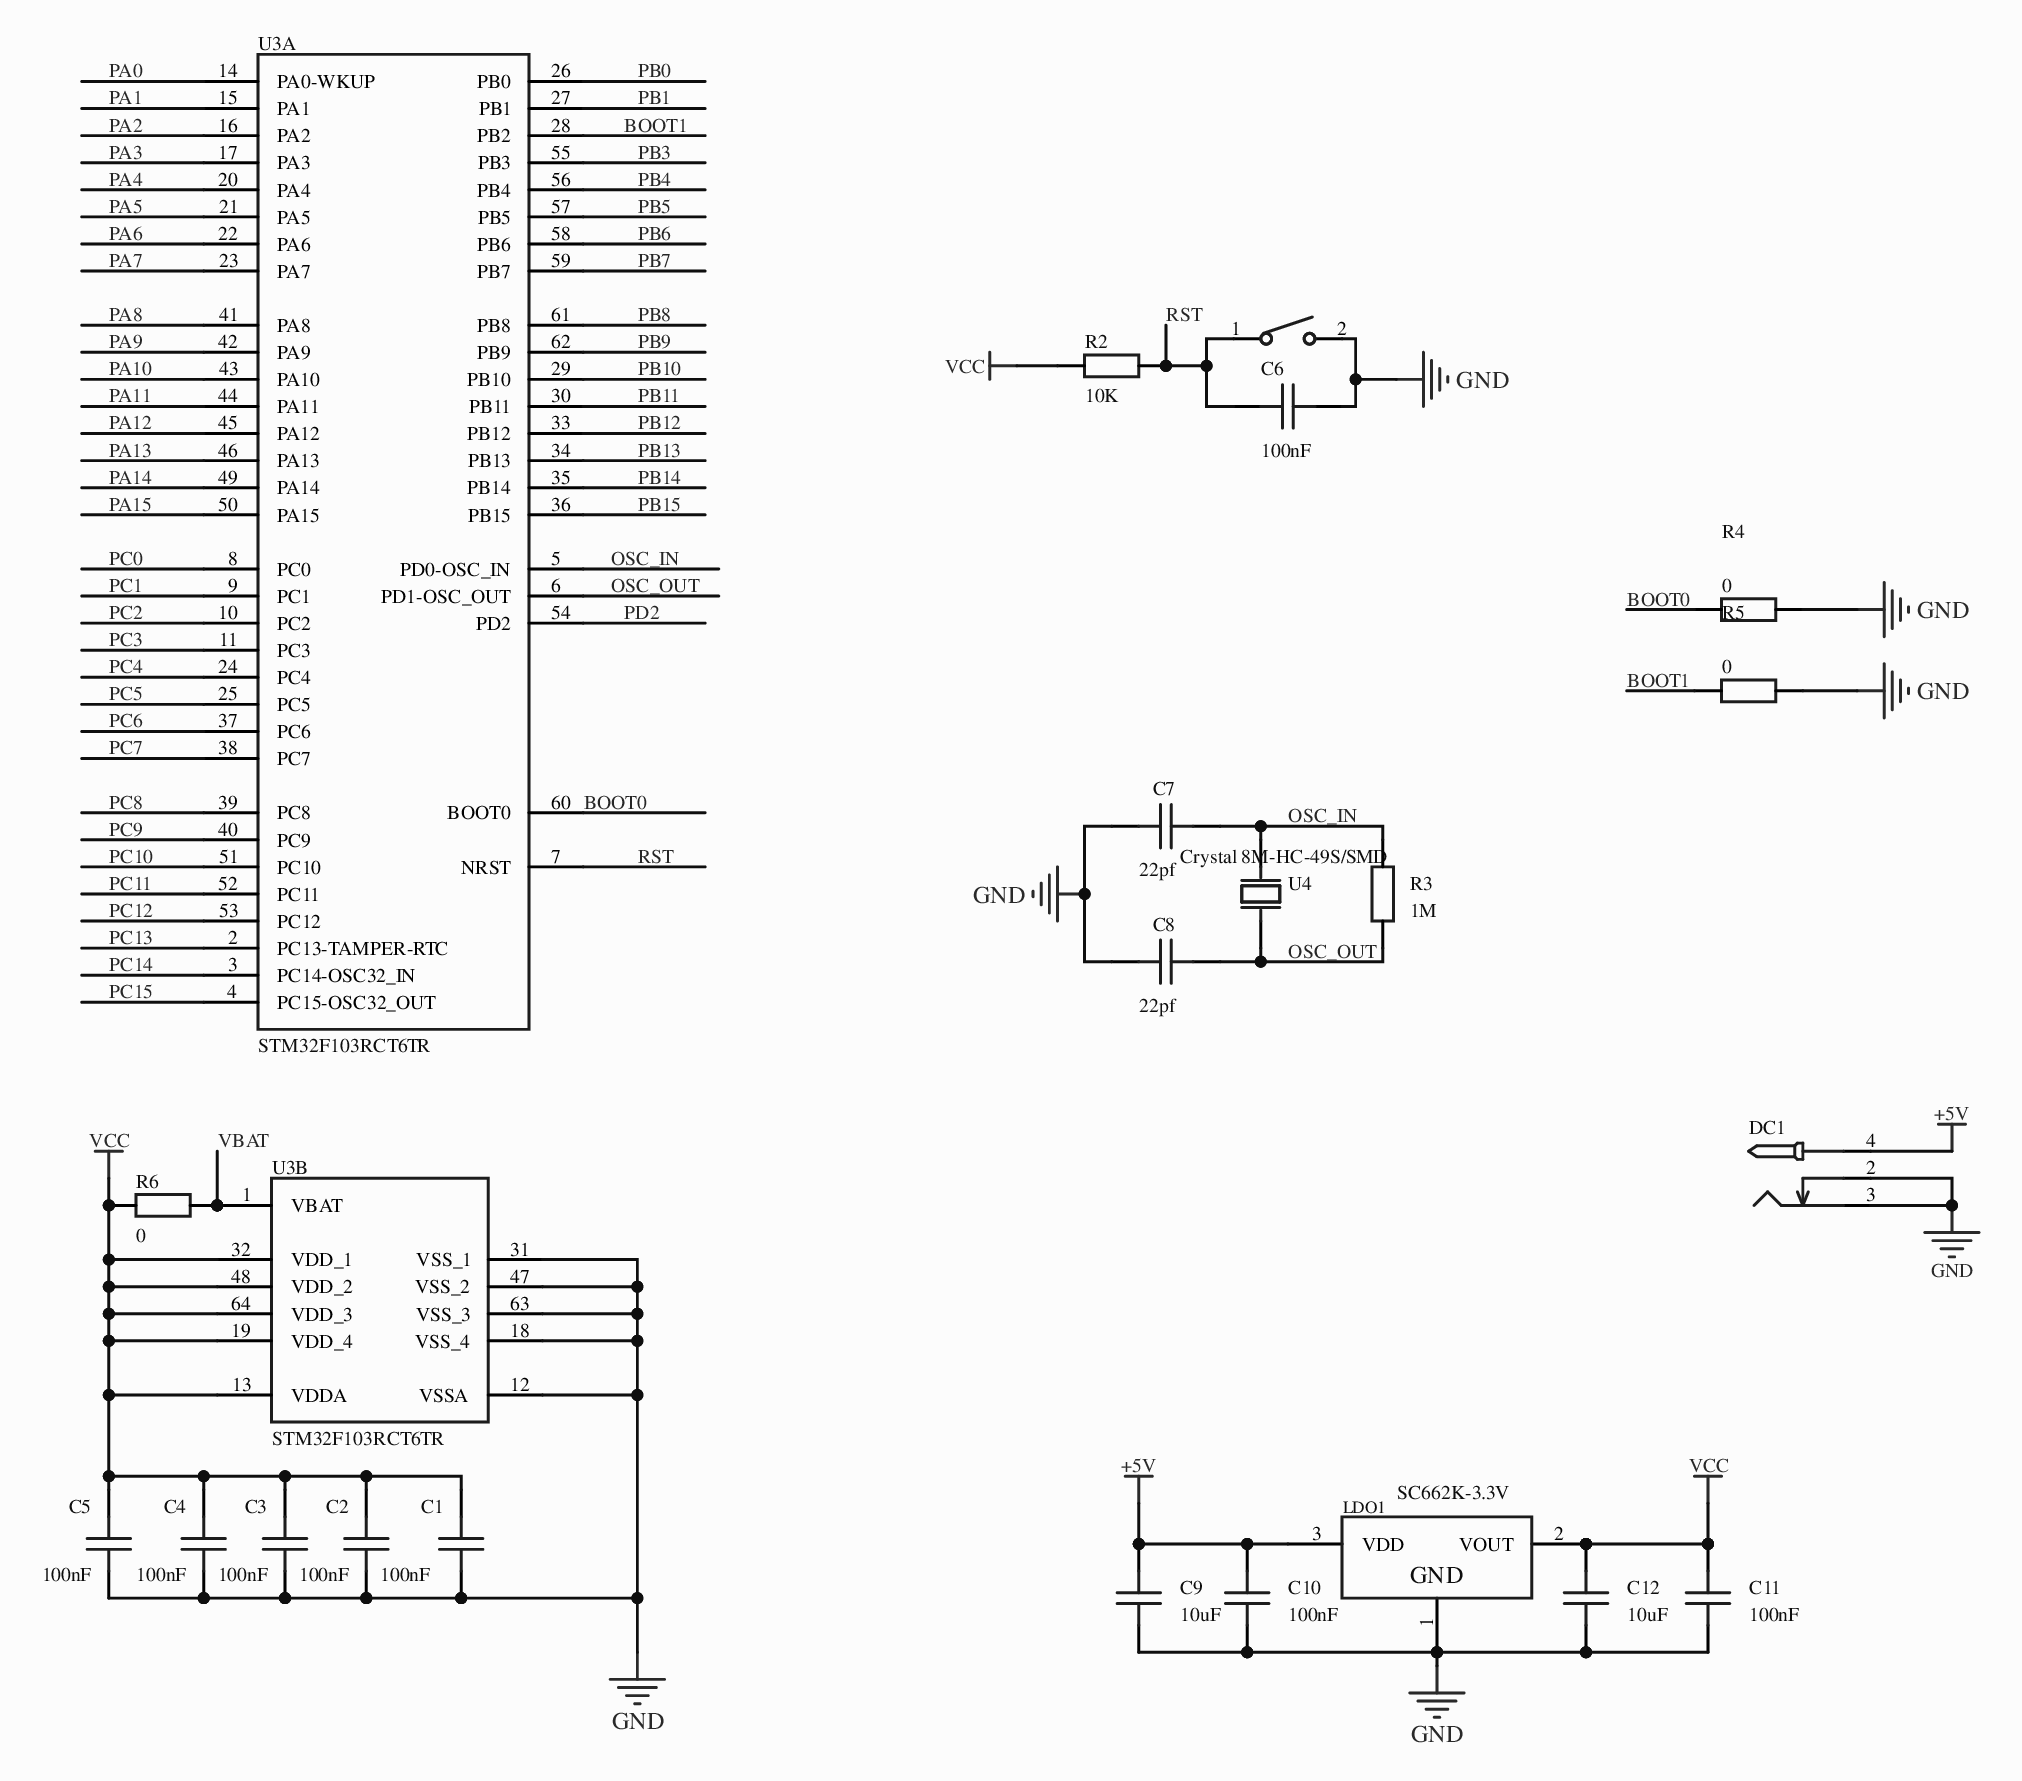
[diagram p0: MISC52126-3.schdoc]
# Altium project MISC52126-2.PrjPcb
1 sheet, 22 parts. Net scope: global (net labels, ports and power ports of the same name join across sheets).
Board file: MISC52126.pcbdoc

## Sheet MISC52126-3.schdoc
size 297 x 209 mm; @Project Name: MISC52126; @Page Count: 1; @Update Date: 2026-05-07; @Create Date: 2026-05-07; @Schematic Name: MISC52126; @Page No: 1

### Parts
C1  100nF  [C0603]
C2  100nF  [C0603]
C3  100nF  [C0603]
C4  100nF  [C0603]
C5  100nF  [C0603]
C6  100nF  [C0603]
C7  22pf  [C0603]
C8  22pf  [C0603]
C9  10uF  [C0603]
C10  100nF  [C0603]
C11  100nF  [C0603]
C12  10uF  [C0603]
DC1  (no value)  [DC-2.0]
LDO1  SC662K-3.3V  [SOT-23-3_L2.9-W1.3-P1.90-LS2.4-BR]
R2  10K  [R0603]
R3  1M  [R0603]
R4  0  [R0603]
R5  0  [R0603]
R6  0  [R0603]
SW1  SMD push button ANJIAN_2PIN  [SW-SMD_L6.0-W3.6-LS8.0]  (value not drawn)
U3  STM32F103RCT6TR  [LQFP-64_L10.0-W10.0-P0.50-LS12.0-BL]  (parts A,B of 2)
U4  Crystal 8M-HC-49S/SMD  [HC-49S_L11.4-W4.8-LS12.7]

### Nets
+5V: C9.2 C10.2 DC1.4 LDO1.3(VDD)
GND: C1.2 C2.2 C3.2 C4.2 C5.2 C6.2 C7.1 C8.1 C9.1 C10.1 C11.1 C12.1 DC1.2 DC1.3 LDO1.1(GND) R4.2 R5.2 SW1.2 U3.12(VSSA) U3.18(VSS_4) U3.31(VSS_1) U3.47(VSS_2) U3.63(VSS_3)
VCC: C1.1 C2.1 C3.1 C4.1 C5.1 C11.2 C12.2 LDO1.2(VOUT) R2.1 R6.1 U3.13(VDDA) U3.19(VDD_4) U3.32(VDD_1) U3.48(VDD_2) U3.64(VDD_3)
BOOT0: R4.1 U3.60(BOOT0)
BOOT1: R5.1 U3.28(PB2)
OSC_IN: C7.2 R3.2 U3.5(PD0-OSC_IN) U4.1(OSC1)
OSC_OUT: C8.2 R3.1 U3.6(PD1-OSC_OUT) U4.2(OSC2)
PA0: U3.14(PA0-WKUP)
PA1: U3.15(PA1)
PA2: U3.16(PA2)
PA3: U3.17(PA3)
PA4: U3.20(PA4)
PA5: U3.21(PA5)
PA6: U3.22(PA6)
PA7: U3.23(PA7)
PA8: U3.41(PA8)
PA9: U3.42(PA9)
PA10: U3.43(PA10)
PA11: U3.44(PA11)
PA12: U3.45(PA12)
PA13: U3.46(PA13)
PA14: U3.49(PA14)
PA15: U3.50(PA15)
PB0: U3.26(PB0)
PB1: U3.27(PB1)
PB3: U3.55(PB3)
PB4: U3.56(PB4)
PB5: U3.57(PB5)
PB6: U3.58(PB6)
PB7: U3.59(PB7)
PB8: U3.61(PB8)
PB9: U3.62(PB9)
PB10: U3.29(PB10)
PB11: U3.30(PB11)
PB12: U3.33(PB12)
PB13: U3.34(PB13)
PB14: U3.35(PB14)
PB15: U3.36(PB15)
PC0: U3.8(PC0)
PC1: U3.9(PC1)
PC2: U3.10(PC2)
PC3: U3.11(PC3)
PC4: U3.24(PC4)
PC5: U3.25(PC5)
PC6: U3.37(PC6)
PC7: U3.38(PC7)
PC8: U3.39(PC8)
PC9: U3.40(PC9)
PC10: U3.51(PC10)
PC11: U3.52(PC11)
PC12: U3.53(PC12)
PC13: U3.2(PC13-TAMPER-RTC)
PC14: U3.3(PC14-OSC32_IN)
PC15: U3.4(PC15-OSC32_OUT)
PD2: U3.54(PD2)
RST: C6.1 R2.2 SW1.1 U3.7(NRST)
VBAT: R6.2 U3.1(VBAT)

### Library data of the parts
C1-C5 = CAP_0603: ConvertToPcb: yes; SymbolName: CapAcitance; ModelId: ac125912035d415993ca9572d50418b1; ModelName: C0603_L1.6-W0.8-H0.8; ModelTransform: 62.992,31.496,0,0,0,0,0,0,0; Device: CAP_0603; AddInBom: yes; Supplier Footprint: 0603; FootprintName: C0603; Value: 100nF
C6-C8 = CAP_0603: Symbol: CapAcitance; ConvertToPcb: yes; ModelId: ac125912035d415993ca9572d50418b1; ModelName: C0603_L1.6-W0.8-H0.8; ModelTransform: 62.992,31.496,0,0,0,0,0,0,0; Device: CAP_0603; AddInBom: yes; Supplier Footprint: 0603; FootprintName: C0603
  C6: Value: 100nF
  C7 C8: Value: 22pf
C9 C12 = CL10A106KP8NNNC: Capacitance:10uF;Tolerance:±10%;Rated voltage:10V;Dielectric (temp. coefficient):X5R;; Manufacturer: SAMSUNG(三星); 3D Model: ac125912035d415993ca9572d50418b1; 3D Model Transform: 62.992,31.496,0,0,0,0,0,0,0; Tolerance: ±10%; Voltage Rated: 10V; Temperature Coefficient: X5R; AddInBom: yes; ModelName: C0603_L1.6-W0.8-H0.8; Symbol: CL10A106KP8NNNC; Device: CL10A106KP8NNNC; LCSC Part Name: 10uF ±10% 10V; Supplier Part: C19702; Manufacturer Part: CL10A106KP8NNNC; Supplier Footprint: 0603; JLCPCB Part Class: Basic library; Datasheet: https://example.com/20160103/1457707703378.pdf; Supplier: LCSC; Value: 10uF; ConvertToPcb: yes; FootprintName: C0603
C10 C11 = CC0603KRX7R9BB104: Capacitance:100nF;Tolerance:±10%;Rated voltage:50V;Dielectric (temp. coefficient):X7R;; Manufacturer: YAGEO(国巨); 3D Model: ac125912035d415993ca9572d50418b1; 3D Model Transform: 62.992,31.496,0,0,0,0,0,0,0; Tolerance: ±10%; Voltage Rated: 50V; Temperature Coefficient: X7R; AddInBom: yes; ModelName: C0603_L1.6-W0.8-H0.8; Symbol: CC0603KRX7R9BB104; Device: CC0603KRX7R9BB104; LCSC Part Name: 100nF ±10% 50V; Supplier Part: C14663; Manufacturer Part: CC0603KRX7R9BB104; Supplier Footprint: 0603; JLCPCB Part Class: Basic library; Datasheet: https://example.com/20180910/C282072_33301C7F631E79921B82A8DAC6BCC5B3.pdf; Supplier: LCSC; Value: 100nF; ConvertToPcb: yes; FootprintName: C0603
DC1 = DC-005_2.0: Symbol: DC power jack; ConvertToPcb: yes; ModelId: f5f20b8a2308479b936ba3c2698865bb0819f05c4eef4c71ace90d822a990e87; ModelName: DC-IN-TH_DC-5520-1; ModelTransform: 372.05,551.18,582.68,90,0,0,137.8,0,-149.61; Device: DC-005_2.0; AddInBom: yes; Supplier Footprint: 插件; FootprintName: DC-2.0
LDO1 = SC662K-3.3V: Output type:Fixed;Output polarity:Positive;Max input voltage:6V;Output voltage:3.3V;Output current:250mA;Power supply ripple rejection (PSRR):50dB@(1kHz);; Manufacturer: FM(富满); 3D Model: c62791f0466c4ae2a892c056b845b0ca; 3D Model Transform: 98.425,114.173,0,180,0,0,0.0005,-0.0005,0; Output Type: Fixed; Number of Outputs: 1; Maximum Input Voltage: 6V; Output Voltage: 3.3V; Dropout Voltage: 38mV@(10mA); Output Current: 250mA; AddInBom: yes; ModelName: SOT-23-3P_L2.9-W1.3-H1.0-LS2.4-P0.95; Symbol: SC662K-3.3V; Device: SC662K-3.3V; LCSC Part Name: 输入6V 输出3.3V 250mA 停产; Supplier Footprint: SOT-23; Datasheet: https://example.com/20161024/1477288576049.pdf; Output Polarity: Positive; Power Supply Rejection Ratio (PSRR): 50dB@(1kHz); Supplier: LCSC; Manufacturer Part: SC662K-3.3V; Supplier Part: C83932; JLCPCB Part Class: Extended library; ConvertToPcb: yes; FootprintName: SOT-23-3_L2.9-W1.3-P1.90-LS2.4-BR
R2-R6 = Res_0603: Symbol: Resistor; ConvertToPcb: yes; ModelId: fc143cca1e79419f9cd78b61e9279f08; ModelTransform: 31.8897,63.7794,0,90,0,0,0,0,0; Device: Res_0603; AddInBom: yes; Supplier Footprint: 0603; FootprintName: R0603; ModelName: R0603
  R2: Value: 10K
  R3: Value: 1M
  R4-R6: Value: 0
SW1 = 贴片按键ANJIAN_2PIN: AddInBom: yes; ModelId: 5cda64a5897044e48badc24f5aa7d420; ModelName: SW-SMD_L6.0-W3.6-H2.5-LS8.0; ModelTransform: 314.96,141.732,0,0,0,0,0,0,0; Symbol: SMD push button ANJIAN_2PIN; Device: SMD push button ANJIAN_2PIN; LCSC Part Name: 贴片按键ANJIAN_2PIN; SupplierPart: C9900015641; ManufacturerPart: 贴片按键ANJIAN_2PIN; Supplier Footprint: SMD-2P; JLCPCB Part Class: Extended library; Supplier: LCSC; ConvertToPcb: yes; FootprintName: SW-SMD_L6.0-W3.6-LS8.0
U3 = STM32F103RCT6TR: CPU core:ARM Cortex-M3;Max CPU frequency:72MHz;Program storage capacity:256KB;Program memory type:FLASH;Total RAM:48KB;GPIO ports:51;; Manufacturer: ST(意法半导体); AddInBom: yes; ModelId: cd9de06618c44fcf82654c43a457f83c; ModelName: LQFP-64_L10.0-W10.0-H1.4-LS12.0-P0.50; ModelTransform: 472.441,472.441,0,0,0,0,0,0,0; CPU Maximum Speed: 72MHz; Operating Voltage Range: 2V~3.6V; Program Storage Size: 256KB; Program Memory Type: FLASH; RAM Size: 48KB; GPIO Ports Number: 51; ADC (Bit): 12bit; Peripheral/Function: Watchdog; DMA; Watchdog; On-chip temperature sensor; Symbol: STM32F103RCT6TR; Device: STM32F103RCT6TR; LCSC Part Name: ARM Cortex-M3 72MHz; SupplierPart: C39704; ManufacturerPart: STM32F103RCT6TR; Supplier Footprint: LQFP-64(10x10); JLCPCB Part Class: Extended Part; Datasheet: https://example.com/20151012/1457707442737.pdf; Supplier: LCSC; ConvertToPcb: yes; FootprintName: LQFP-64_L10.0-W10.0-P0.50-LS12.0-BL; CPU Core: ARM Cortex-M3; EEPROM: -; DAC (Bit): 12bit; PWM (Bit): -; Universal Serial Bus: Yes; Internal Comparator: -; communication protocol: -; Watchdog: Yes; Real-Time Clock: -; Infrared Data Association: Yes; Low-Voltage Detect: Yes; CCP Capture/Compare: -; Secure Digital Input and Output: -; Direct Memory Access: Yes; Internal Oscillator: Yes; Operating Temperature Range: -40℃~+85℃
U4 = 晶振8M-HC-49S/SMD: AddInBom: yes; ModelId: 6f569b91267b44029b8615eb5c810fba; ModelName: HC-49S_L11.4-W1.8-H3.0-LS12.7; ModelTransform: 499.999,188.976,0,0,0,0,0.0005,0,0; Symbol: Crystal 8M-HC-49S/SMD; Device: Crystal 8M-HC-49S/SMD; LCSC Part Name: 晶振8M-HC-49S/SMD; SupplierPart: C9900009291; ManufacturerPart: 晶振8M-HC-49S/SMD; Supplier Footprint: SMD; JLCPCB Part Class: Extended library; Supplier: LCSC; ConvertToPcb: yes; FootprintName: HC-49S_L11.4-W4.8-LS12.7